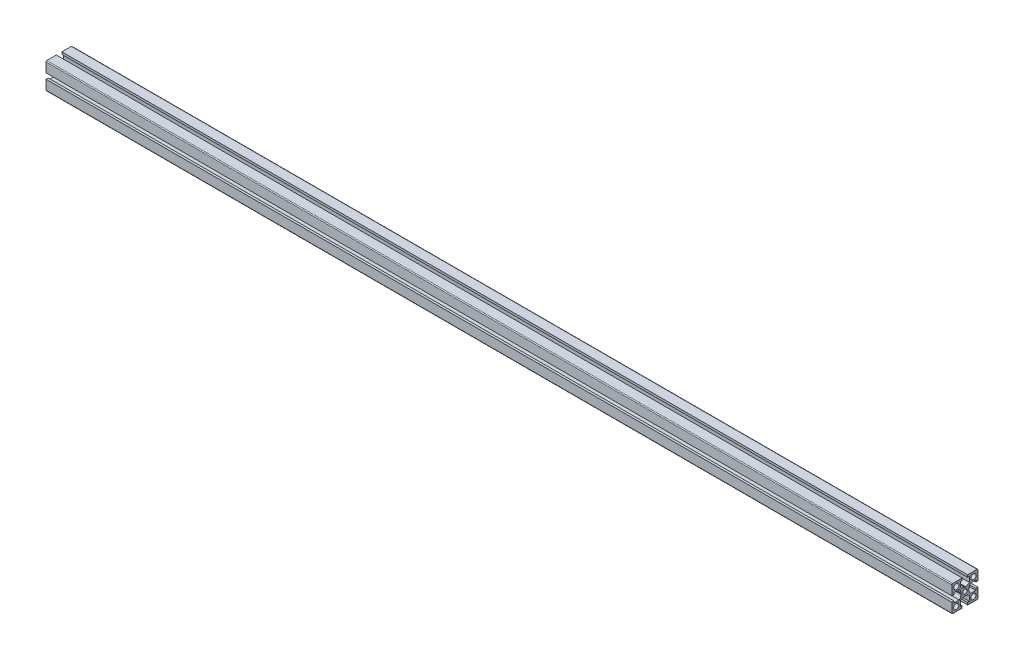
SolidWorks part; units mm, degrees
ref_plane "前视基准面" through (0, 0, 0) normal (0, 0, 1) x (1, 0, 0)
ref_plane "上视基准面" through (0, 0, 0) normal (0, 1, 0) x (1, 0, 0)
ref_plane "右视基准面" through (0, 0, 0) normal (1, 0, 0) x (0, 0, -1)
sketch "草图1" plane through (0, 0, 0) normal (0, 1, 0) x (1, 0, 0)
  line L0 (0, 0) -> (1040, 0)
  dimension "D1" = 1040
other "0国耀铝型材 GY-3030国标铝型材(1)"
ref_plane "基准面1" through (0, 0, 0) normal (1, 0, 0) x (0, 0, -1)
sketch "草图11" plane through (0, 0, 0) normal (1, 0, 0) x (0, 0, -1)
  line L0 (0, 0) -> (15, 0) construction
  line L1 (0, 0) -> (0, 15) construction
  line L42 (-14, -15) -> (-3.15, -15)
  line L43 (-3.15, -15) -> (-3.15, -12.5)
  line L44 (-3.15, -12.5) -> (-5.15, -12.5)
  line L45 (-5.15, -12.5) -> (-5.15, -6.5)
  line L46 (-0.555, -4.52) -> (0, -4.2)
  line L47 (0, -4.2) -> (0.555, -4.52)
  line L48 (5.15, -6.5) -> (5.15, -12.5)
  line L49 (5.15, -12.5) -> (3.15, -12.5)
  line L50 (3.15, -12.5) -> (3.15, -15)
  line L51 (3.15, -15) -> (14, -15)
  line L52 (15, -14) -> (15, -3.15)
  line L53 (15, -3.15) -> (12.5, -3.15)
  line L54 (12.5, -3.15) -> (12.5, -5.15)
  line L55 (12.5, -5.15) -> (6.5, -5.15)
  line L56 (4.52, -0.554) -> (4.2, 0)
  line L57 (4.2, 0) -> (4.52, 0.555)
  line L58 (6.5, 5.15) -> (12.5, 5.15)
  line L59 (12.5, 5.15) -> (12.5, 3.15)
  line L60 (12.5, 3.15) -> (15, 3.15)
  line L61 (15, 3.15) -> (15, 14)
  line L62 (14, 15) -> (3.15, 15)
  line L63 (3.15, 15) -> (3.15, 12.5)
  line L64 (3.15, 12.5) -> (5.15, 12.5)
  line L65 (5.15, 12.5) -> (5.15, 6.5)
  line L66 (0.555, 4.521) -> (0, 4.2)
  line L67 (0, 4.2) -> (-0.555, 4.521)
  line L68 (-5.15, 6.5) -> (-5.15, 12.5)
  line L69 (-5.15, 12.5) -> (-3.15, 12.5)
  line L70 (-3.15, 12.5) -> (-3.15, 15)
  line L71 (-3.15, 15) -> (-14, 15)
  line L72 (-15, 14) -> (-15, 3.15)
  line L73 (-15, 3.15) -> (-12.5, 3.15)
  line L74 (-12.5, 3.15) -> (-12.5, 5.15)
  line L75 (-12.5, 5.15) -> (-6.5, 5.15)
  line L76 (-4.52, 0.555) -> (-4.2, 0)
  line L77 (-4.2, 0) -> (-4.52, -0.554)
  line L78 (-6.5, -5.15) -> (-12.5, -5.15)
  line L79 (-12.5, -5.15) -> (-12.5, -3.15)
  line L80 (-12.5, -3.15) -> (-15, -3.15)
  line L81 (-15, -3.15) -> (-15, -14)
  arc A13 (-15, -14) -> (-14, -15) centre (-14, -14) ccw
  arc A14 (-5.15, -6.5) -> (-0.555, -4.52) centre (0.0004, -12.1308) cw
  arc A15 (0.555, -4.52) -> (5.15, -6.5) centre (-0.0004, -12.1308) cw
  arc A16 (14, -15) -> (15, -14) centre (14, -14) ccw
  arc A17 (6.5, -5.15) -> (4.52, -0.554) centre (12.1308, 0.0003) cw
  arc A18 (4.52, 0.555) -> (6.5, 5.15) centre (12.1308, -0.0004) cw
  arc A19 (15, 14) -> (14, 15) centre (14, 14) ccw
  arc A20 (5.15, 6.5) -> (0.555, 4.521) centre (0.0008, 12.1318) cw
  arc A21 (-0.555, 4.521) -> (-5.15, 6.5) centre (-0.0008, 12.1318) cw
  arc A22 (-14, 15) -> (-15, 14) centre (-14, 14) ccw
  arc A23 (-6.5, 5.15) -> (-4.52, 0.555) centre (-12.1308, -0.0004) cw
  arc A24 (-4.52, -0.554) -> (-6.5, -5.15) centre (-12.1308, 0.0003) cw
  circle A25 centre (9.8, 9.9) radius 3
  circle A26 centre (9.8, -9.9) radius 3
  circle A27 centre (0, 0) radius 2.5
  circle A28 centre (-9.8, 9.9) radius 3
  circle A29 centre (-10, -9.9) radius 3
  point P0 (0, 0)
  dimension "D3" = 19.8
  dimension "D2" = 19.8
  dimension "D5" = 5
  dimension "D6" = 6
  dimension "D4" = 6.3
  dimension "D9" = 30
  dimension "D10" = 30
